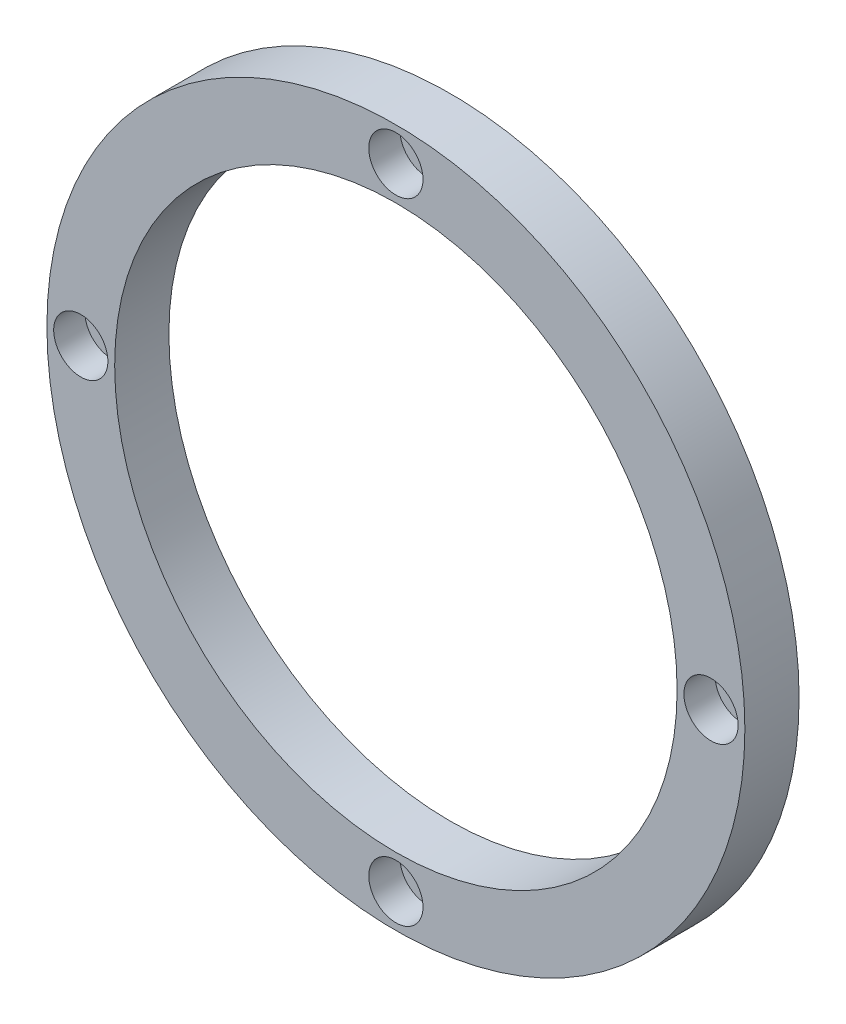
from build123d import *

# Parameters (mm, degrees)
SKETCH1_R           = 51.5
SKETCH1_R_2         = 41.5
BOSS_EXTRUDE1_DEPTH = 8
CIRPATTERN1_COUNT   = 4


with BuildPart() as part:
    # Sketch1 → Boss-Extrude1 (new body)
    with BuildSketch(Plane.XY):
        Circle(SKETCH1_R)
        Circle(SKETCH1_R_2, mode=Mode.SUBTRACT)
    extrude(amount=BOSS_EXTRUDE1_DEPTH)

    # Sketch5 → Hole size per hex socket cap screw type1 (revolve, cut)
    with BuildSketch(Plane(origin=(0, 46.5, 8), x_dir=(0, -1, 0), z_dir=(1, 0, 0))):
        Polygon((0, 0), (0, 18.351936393), (2.25, 17), (2.25, 4.6), (4, 4.6), (4, 0), align=None)
    hole_size_per_hex_socket_cap_screw_type1 = revolve(axis=Axis((0, 46.5, 14.35), (0, 0, -1)), mode=Mode.SUBTRACT)

    # CirPattern1: Hole size per hex socket cap screw type1 ×4 about axis
    cirpattern1_axis = Axis((0, 0, 0), (0, 0, 1))
    for i in range(1, CIRPATTERN1_COUNT):
        add(hole_size_per_hex_socket_cap_screw_type1.rotate(cirpattern1_axis, i * 360 / CIRPATTERN1_COUNT), mode=Mode.SUBTRACT)


solid = part.part
